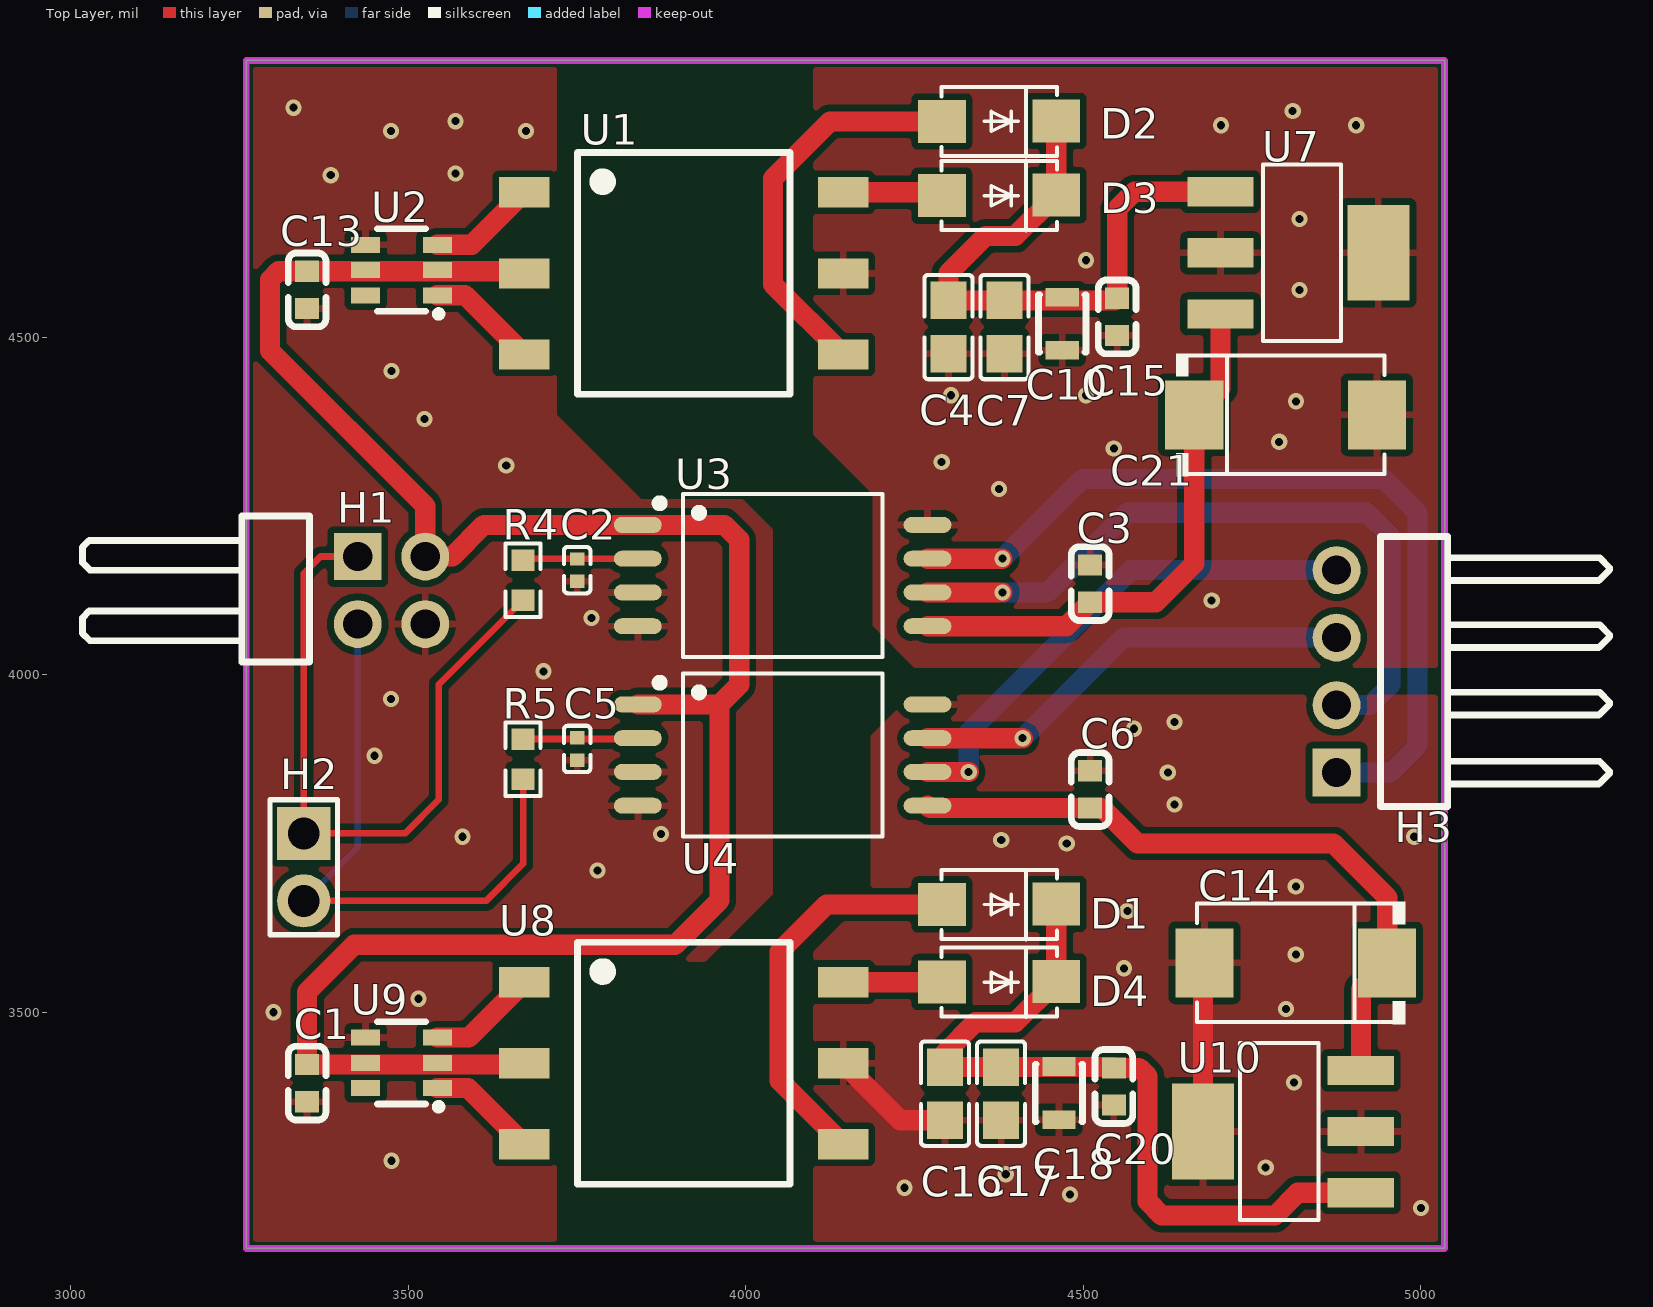
[diagram p0: Top Layer view]
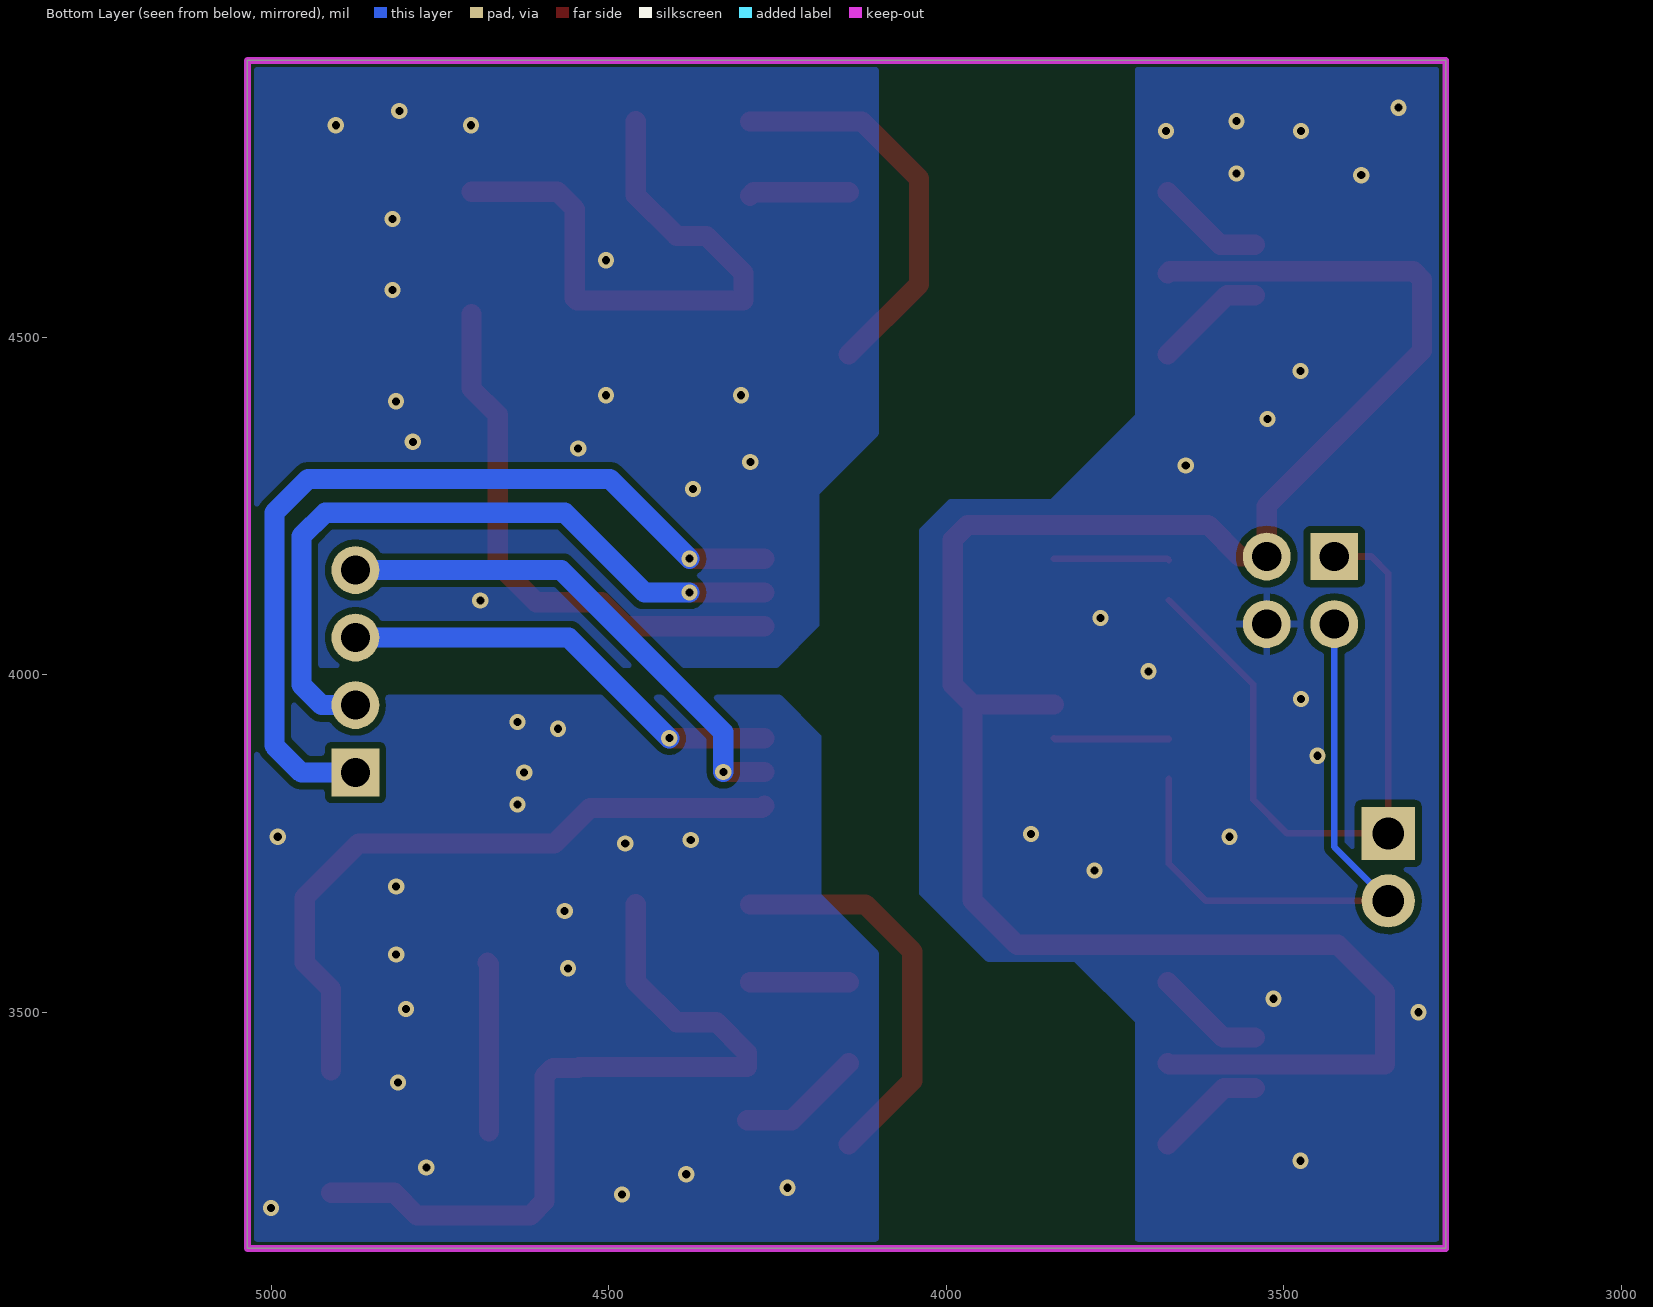
[diagram p1: Bottom Layer view, seen from below]
# Altium PCB MISC51425.pcbdoc
Units mil, origin at the board's own origin, x right, y up, seen from the top; angles counter-clockwise.
Board outline 1775 x 1760 mil, 2 copper layers (Top Layer, Bottom Layer), stack 2.757 mil thick; 33 components, 24 nets, 102 pads, 55 vias.

## Layer stack, top to bottom
Top Solder Mask Layer: solder mask 0.394, Dk 3.3
Top Layer: signal copper 1.379
Bottom Layer: signal copper 1.378
Bottom Solder Mask Layer: solder mask 0.394, Dk 3.3

## Board outline
3260,4910 3260,3150 5035,3150 5035,4910

## Design rules (kind name [scope] priority, off if disabled: settings)
BoardOutlineClearance Plane_innerPlane_1 [All] p2 off: genericclearance=4 ignorepadtopadclearanceinfootprint=FALSE except(0: Arc-SplitContinuation Track-SplitContinuation SMDPad-SplitContinuation THPad-SplitContinuation Via-SplitContinuation Fill-SplitContinuation Region-SplitContinuation Poly-SplitContinuation Text-SplitContinuation Hole-SplitContinuation; 6: Arc-CutoutEdge Track-CutoutEdge SMDPad-CutoutEdge THPad-CutoutEdge Via-CutoutEdge Text-CutoutEdge; 6.9: Hole-OutlineEdge Hole-CutoutEdge; 10: Poly-OutlineEdge Poly-CutoutEdge; 11.8: Arc-OutlineEdge Track-OutlineEdge SMDPad-OutlineEdge THPad-OutlineEdge Via-OutlineEdge Fill-OutlineEdge Region-OutlineEdge Text-OutlineEdge Fill-CutoutEdge Region-CutoutEdge)
BoardOutlineClearance Copper_copperRegion_1 [All] p4 off: genericclearance=4 ignorepadtopadclearanceinfootprint=FALSE except(0: Arc-SplitContinuation Track-SplitContinuation SMDPad-SplitContinuation THPad-SplitContinuation Via-SplitContinuation Fill-SplitContinuation Region-SplitContinuation Poly-SplitContinuation Text-SplitContinuation Hole-SplitContinuation; 6: Arc-CutoutEdge Track-CutoutEdge SMDPad-CutoutEdge THPad-CutoutEdge Via-CutoutEdge Text-CutoutEdge; 6.9: Hole-OutlineEdge Hole-CutoutEdge; 10: Poly-OutlineEdge Poly-CutoutEdge; 11.8: Arc-OutlineEdge Track-OutlineEdge SMDPad-OutlineEdge THPad-OutlineEdge Via-OutlineEdge Fill-OutlineEdge Region-OutlineEdge Text-OutlineEdge Fill-CutoutEdge Region-CutoutEdge)
BoardOutlineClearance copperThickness1oz_1 [All] p6: genericclearance=4 ignorepadtopadclearanceinfootprint=FALSE except(0: Arc-SplitContinuation Track-SplitContinuation SMDPad-SplitContinuation THPad-SplitContinuation Via-SplitContinuation Fill-SplitContinuation Region-SplitContinuation Poly-SplitContinuation Text-SplitContinuation Hole-SplitContinuation; 6: Arc-CutoutEdge Track-CutoutEdge SMDPad-CutoutEdge THPad-CutoutEdge Via-CutoutEdge Text-CutoutEdge; 6.9: Hole-OutlineEdge Hole-CutoutEdge; 10: Poly-OutlineEdge Poly-CutoutEdge; 11.8: Arc-OutlineEdge Track-OutlineEdge SMDPad-OutlineEdge THPad-OutlineEdge Via-OutlineEdge Fill-OutlineEdge Region-OutlineEdge Text-OutlineEdge Fill-CutoutEdge Region-CutoutEdge)
Clearance Plane_innerPlane [All] p1 off: gap=4 ignorepadtopadclearanceinfootprint=FALSE except(6: SMDPad-Track SMDPad-SMDPad THPad-Track SMDPad-THPad THPad-THPad Track-Via SMDPad-Via THPad-Via Via-Via Fill-SMDPad Region-SMDPad Fill-THPad Region-THPad Fill-Via Region-Via Fill-Fill Fill-Region Region-Region Arc-Track Arc-SMDPad Arc-THPad Arc-Via Fill-Arc Region-Arc Arc-Arc Text-Track SMDPad-Text Text-THPad Text-Via Fill-Text Region-Text Arc-Text Text-Text; 6.9: Hole-Track Hole-SMDPad Hole-THPad Hole-Via Fill-Hole Region-Hole Hole-Arc Hole-Text; 10: Poly-Track Poly-SMDPad Poly-THPad Poly-Via Poly-Fill Poly-Region Poly-Poly Poly-Arc Poly-Text Poly-Hole; 11.8: Fill-Track Region-Track)
Clearance Copper_copperRegion [All] p3 off: gap=4 ignorepadtopadclearanceinfootprint=FALSE except(6: SMDPad-Track SMDPad-SMDPad THPad-Track SMDPad-THPad THPad-THPad Track-Via SMDPad-Via THPad-Via Via-Via Fill-SMDPad Region-SMDPad Fill-THPad Region-THPad Fill-Via Region-Via Fill-Fill Fill-Region Region-Region Arc-Track Arc-SMDPad Arc-THPad Arc-Via Fill-Arc Region-Arc Arc-Arc Text-Track SMDPad-Text Text-THPad Text-Via Fill-Text Region-Text Arc-Text Text-Text; 6.9: Hole-Track Hole-SMDPad Hole-THPad Hole-Via Fill-Hole Region-Hole Hole-Arc Hole-Text; 10: Poly-Track Poly-SMDPad Poly-THPad Poly-Via Poly-Fill Poly-Region Poly-Poly Poly-Arc Poly-Text Poly-Hole; 11.8: Fill-Track Region-Track)
Clearance copperThickness1oz [All] p5: gap=4 ignorepadtopadclearanceinfootprint=FALSE except(6: SMDPad-Track SMDPad-SMDPad THPad-Track SMDPad-THPad THPad-THPad Track-Via SMDPad-Via THPad-Via Via-Via Fill-SMDPad Region-SMDPad Fill-THPad Region-THPad Fill-Via Region-Via Fill-Fill Fill-Region Region-Region Arc-Track Arc-SMDPad Arc-THPad Arc-Via Fill-Arc Region-Arc Arc-Arc Text-Track SMDPad-Text Text-THPad Text-Via Fill-Text Region-Text Arc-Text Text-Text; 6.9: Hole-Track Hole-SMDPad Hole-THPad Hole-Via Fill-Hole Region-Hole Hole-Arc Hole-Text; 10: Poly-Track Poly-SMDPad Poly-THPad Poly-Via Poly-Fill Poly-Region Poly-Poly Poly-Arc Poly-Text Poly-Hole; 11.8: Fill-Track Region-Track)
DiffPairsRouting differentialPair [All] p1: maxlimit=6 minlimit=5 mostfreqgap=6 toplayer_minwidth=5 toplayer_prefwidth=100 toplayer_maxwidth=100 toplayer_mingap=5 toplayer_prefgap=6 toplayer_maxgap=6 bottomlayer_minwidth=5 bottomlayer_prefwidth=100 bottomlayer_maxwidth=100 bottomlayer_mingap=5 bottomlayer_prefgap=6 bottomlayer_maxgap=6 maxuncoupledlength=10
HoleToHoleClearance otherClearance [All] p1: gap=11.8 allowstackedmicrovias=TRUE
Length netLength [All] p1: minlimit=0 maxlimit=0
MatchedLengths netLengthTolerance [All] p1: tolerance=1000
PasteMaskExpansion pasteMaskExpansion [All] p1: expansion=0
PlaneConnect innerPlane [All] p1: planeconnectstyle=Relief reliefexpansion=20 reliefentries=4 reliefconductorwidth=10 reliefairgap=10
PolygonConnect copperRegion [(InNet('SGND') OR InNet('$1N9') OR InNet('$1N10'))] p1: connectstyle=Relief reliefconductorwidth=10 reliefentries=4 polygonreliefangle="90 Angle" airgapwidth=10 via.connectstyle=Relief via.reliefconductorwidth=10 via.reliefentries=4 via.polygonreliefangle="90 Angle" via.airgapwidth=10
RoutingVias viaSize [All] p1: holewidth=12.01 width=24.02 viastyle="Through Hole" minholewidth=11.81 minwidth=19.68 maxholewidth=248.03 maxwidth=393.7
SolderMaskExpansion solderMaskExpansion [IsVia] p1: expansion=-1000 istentingtop=TRUE
SolderMaskExpansion solderMaskExpansion [All] p2: expansion=2 istentingtop=FALSE
Width copperThickness1oz_2 [All] p1: maxlimit=100 minlimit=5 preferedwidth=10

## Components (designator, comment, footprint, x,y, rotation, side; value= is the part's Value field where it differs from the comment)
C1 "10uF" C0603 3350,3395 r270 top
C2 "22pF" C0402 3750,4155 r90 top
C3 "100nF" C0603 4510,4135 r270 top
C4 "4.7uF" C0805 4300,4515 r90 top
C5 "22pF" C0402 3750,3890 r90 top
C6 "100nF" C0603 4510,3830 r270 top
C7 "4.7uF" C0805 4383.1,4515 r90 top
C10 "100nF" CAP-SMD_L2.0-W1.25 4468.67,4520 r90 top
C13 "100nF" C0603 3350,4570 r270 top
C14 "47uF" CAP-SMD_L7.3-W4.3-FD 4814.68,3573.21 r180 top
C15 "470nF" C0603 4550,4530 r90 top
C16 "4.7uF" C0805 4295,3379.45 r90 top
C17 "4.7uF" C0805 4378.1,3379.45 r90 top
C18 "100nF" CAP-SMD_L2.0-W1.25 4463.67,3380.18 r90 top
C20 "470nF" C0603 4545,3390 r90 top
C21 "47uF" CAP-SMD_L7.3-W4.3-FD 4799.43,4385 r0 top
D1 "SS34" SMA_L4.3-W2.6-LS5.0-FD 4375,3660 r0 top
D2 "SS34" SMA_L4.3-W2.6-LS5.0-FD 4375,4820 r0 top
D3 "SS34" SMA_L4.3-W2.6-LS5.0-FD 4375,4710 r0 top
D4 "SS34" SMA_L4.3-W2.6-LS5.0-FD 4375,3545 r0 top
H1 "PZ254R-12-4P" HDR-TH_4P-P2.54-H-M-R2-C2-S2.54 3475,4125 r270 top
H2 "PZ254V-11-02P" HDR-TH_2P-P2.54-V-M 3345,3715 r270 top
H3 "PZ254R-11-04P" HDR-TH_4P-P2.54-H-M-W10.4 4875,4005 r90 top
R4 "51Ω" R0603 3670,4140 r90 top
R5 "51Ω" R0603 3670,3875 r90 top
U1 "750342879" XFMR-SMD_6P-L9.1-W8.0-P3.05-LS13.0-TL 3907.91,4594.45 r0 top
U2 "SN6505BDBVR" SOT-23-6_L2.9-W1.6-P0.95-LS2.8-BR 3489.8,4599.45 r0 top
U3 "UCC5350MCQDWVRQ1" SOIC-8_L7.5-W5.9-P1.27-LS11.5-BL 4054.57,4146.89 r270 top
U4 "UCC5350MCQDWVRQ1" SOIC-8_L7.5-W5.9-P1.27-LS11.5-BL 4054.57,3880.97 r270 top
U7 "LM2940IMP-15/NOPB" SOT-223-3_L6.5-W3.4-P2.30-LS7.0-BR 4820,4625 r180 top
U8 "750342879" XFMR-SMD_6P-L9.1-W8.0-P3.05-LS13.0-TL 3907.91,3424.45 r0 top
U9 "SN6505BDBVR" SOT-23-6_L2.9-W1.6-P0.95-LS2.8-BR 3489.8,3425 r0 top
U10 "LM2940IMP-15/NOPB" SOT-223-3_L6.5-W3.4-P2.30-LS7.0-BR 4794.11,3323.21 r0 top

## Footprints (in the part's own frame and the unit in brackets; to place one, negate y for a bottom-side part, rotate by r counter-clockwise, add the part's x,y. Pads: shape width x height; smd on the part's side, far side on the other; paste and mask are expansions set on the pad)
C0402 [mm]
  rect 0.5x0.54 smd: 1(-0.42,0) 2(0.42,0)
  silkscreen extent -0.87,-0.5 0.87,0.5
C0603 [mm]
  rect 0.8x0.9 smd: 1(-0.7,0) 2(0.7,0)
  silkscreen extent -1.39,-0.71 1.39,0.71
C0805 [mm]
  rect 1.41x1.35 smd paste-100 mask+0.051: 1(-1,0) 2(1,0)
  silkscreen extent -1.96,-0.9 1.96,0.9
CAP-SMD_L2.0-W1.25 [mm]
  rect 0.7x1.25 smd: 1(-1,0) 2(1,0)
  silkscreen extent -1.08,-0.89 1.08,0.89
CAP-SMD_L7.3-W4.3-FD [mm]
  rect 2.185x2.592 smd: 1(-3.437,0) 2(3.437,0)
  silkscreen extent -4.11,-2.3 3.72,2.3
HDR-TH_2P-P2.54-V-M [mm]
  rect 2x2 hole 1.2: 1(-1.27,0)
  round 2 hole 1.2: 2(1.27,0)
  silkscreen extent -2.54,-1.27 2.54,1.27
HDR-TH_4P-P2.54-H-M-R2-C2-S2.54 [mm]
  rect 1.778x1.8 hole 1.1: 1(-1.27,-1.27)
  round 1.8 hole 1.1: 2(-1.27,1.27) 3(1.27,-1.27) 4(1.27,1.27)
  silkscreen extent -2.79,-11.63 2.7,-3.09
HDR-TH_4P-P2.54-H-M-W10.4 [mm]
  rect 1.8x1.8 hole 1.1: 1(-3.81,0)
  round 1.8 hole 1.1: 2(-1.27,0) 3(1.27,0) 4(3.81,0)
  silkscreen extent -5.09,-10.27 5.07,-1.65
R0603 [mil]
  rect 31.75x34.02 smd paste-3937.01 mask+2: 1(-29.66,0) 2(29.66,0)
  silkscreen extent -55,-26 55,26
SMA_L4.3-W2.6-LS5.0-FD [mm]
  rect 1.8x1.62 smd: 1(-2.15,-0.009) 2(2.15,0.009)
  silkscreen extent -2.17,-1.32 2.19,1.29
SOIC-8_L7.5-W5.9-P1.27-LS11.5-BL [mm]
  oval 0.6x1.8 smd: 1(-1.905,-5.45) 2(-0.635,-5.45) 3(0.635,-5.45) 4(1.905,-5.45) 5(1.905,5.45) 6(0.635,5.45) 7(-0.635,5.45) 8(-1.905,5.45)
  silkscreen extent -3.06,-4.78 3.06,3.75
SOT-23-6_L2.9-W1.6-P0.95-LS2.8-BR [mm]
  rect 1.1x0.6 smd paste+0 mask+0.051: 1(1.35,-0.95) 2(1.35,0) 3(1.35,0.95) 4(-1.35,0.95) 5(-1.35,0) 6(-1.35,-0.95)
  silkscreen extent -0.9,-1.78 1.52,1.55
SOT-223-3_L6.5-W3.4-P2.30-LS7.0-BR [mm]
  rect 2.5x1.1 smd: 1(2.97,-2.3) 2(2.97,0) 3(2.97,2.3)
  rect 2.34x3.6 smd: 4(-2.97,0)
  silkscreen extent -1.57,-3.33 1.37,3.33
XFMR-SMD_6P-L9.1-W8.0-P3.05-LS13.0-TL [mm]
  rect 1.9x1.14 smd: 1(-6,3.05) 2(-6,0) 3(-6,-3.05) 4(6,3.05) 5(6,0) 6(6,-3.05)
  silkscreen extent -4,-4.55 4,4.55

## Via types
v1: diameter 24.02, hole 12, Top Layer to Bottom Layer, 55 vias

## Nets (pads, with @x,y where several pads share a name; then routed paths per layer and width w, separated by ;. In a path a pad name is that pad's centre, name@x,y a point inside that pad or via, vN(x,y) a via of type N, cw(c..) or ccw(c..) an arc to the next point about the centre after c; other vN are vias at no path point)
15V: C6.2 C14.1 U4.5 U10.3 | length 1009.6
  Top Layer w30: U4.5 4272.67,3802.44 C6.2 4527.56,3802.44 4580,3750 4870,3750 4949.98,3670.02 C14.1 4911.03,3534.26 U10.3
15V_H: C3.2 C21.1 U3.5 U7.3 | length 819.7
  Top Layer w30: U3.5 4474.45,4071.89 C3.2 4607.44,4107.44 4664.13,4164.13 C21.1 4703.07,4423.95 U7.3
$1N9: C4.2 C7.2 C10.2 C15.2 D2.2 D3.2 U7.1 | length 905.5
  Top Layer w30: D2.2 D3.2 4399.27,4650 4355,4650 4300,4595 C4.2 C7.2 4546.81,4554.37 C15.2 4550,4690 4575.55,4715.55 U7.1
$1N10: C16.2 C17.2 C18.2 C20.2 D1.2 D4.2 U10.1 | length 1174
  Top Layer w30: D1.2 D4.2 4399.27,3485 4340,3485 4295,3440 C16.2 C17.2 4543.74,3418.82 C20.2 4582.44,3417.56 4595,3405 4595,3220 4616.21,3198.79 4783.79,3198.79 4817.66,3232.66 U10.1
$1N15: D4.1 U8.4 | length 146.3
  Top Layer w30: U8.4 4290.25,3544.52 D4.1
$1N16: D3.1 U1.4 | length 148.3
  Top Layer w30: U1.4 4285.46,4714.52 D3.1
$1N17: D2.1 U1.6 | length 589.2
  Top Layer w30: U1.6 4040,4578.5 4040,4735 4124.63,4819.63 D2.1
$1N18: D1.1 U8.6 | length 593.8
  Top Layer w30: U8.6 4050,3398.5 4050,3590 4119.63,3659.63 D1.1
$1N21: U1.3 U2.1 | length 165.1
  Top Layer w30: U2.1 3584.02,4562.05 U1.3
$1N22: U8.3 U9.1 | length 163.2
  Top Layer w30: U9.1 3588.47,3387.6 U8.3
$1N25: U8.1 U9.3 | length 162.8
  Top Layer w30: U9.3 3589.57,3462.4 U8.1
$1N26: U1.1 U2.3 | length 160.9
  Top Layer w30: U2.3 3594.02,4636.85 U1.1
$1N41: C2.2 R4.2 U3.2 | length 170.9
  Top Layer w10: R4.2 3672.23,4171.89 U3.2
$1N42: C5.2 R5.2 U4.2 | length 170.5
  Top Layer w10: R5.2 3838.68,3904.66 U4.2
+5V: C1.1 C13.1 H1.2 U1.2 U2.2 U2.5 U3.1 U4.1 U8.2 U9.2 U9.5 | length 3146.2
  Top Layer w30: U8.2 3669.8,3422.56 C1.1 3350,3530 3420,3600 3895,3600 3960.97,3665.97 3960.97,3955.97 ; U1.2 3668.59,4597.56 C13.1 3307.56,4597.56 3295,4585 3295,4480 3525,4250 H1.2 3565,4175 3611.89,4221.89 U3.1 3968.11,4221.89 3990,4200 3990,3985 3960.97,3955.97 ; U4.1 3960.97,3955.97
CLAMP1_H: H3.1 U3.7 | length 1277.1
  Top Layer w30: U3.7 v1(4380,4171.89)
  Bottom Layer w30: v1(4380,4171.89) 4498.11,4290 4945,4290 4995,4240 4995,3895 4955,3855 H3.1
CLAMP1_L: H3.3 U4.7 | length 667.6
  Top Layer w30: U4.7 v1(4410,3905.97)
  Bottom Layer w30: v1(4410,3905.97) 4559.03,4055 H3.3
G1H: H3.2 U3.6 | length 1061.7
  Top Layer w30: U3.6 v1(4380,4121.89)
  Bottom Layer w30: v1(4380,4121.89) 4446.89,4121.89 4565,4240 4920,4240 4955,4205 4955,3985 4925,3955 H3.2
G1L: H3.4 U4.6 | length 764.3
  Top Layer w30: U4.6 v1(4330,3855.97)
  Bottom Layer w30: v1(4330,3855.97) 4330,3915 4570,4155 H3.4
PWM1: H1.1 H2.1 R4.1 | length 1043.2
  Top Layer w10: H1.1 3370,4175 3345,4150 H2.1 3495,3765 3545,3815 3545,3985.34 R4.1
PWM2: H1.3 H2.2 R5.1 | length 916.3
  Top Layer w10: H2.2 3615,3665 3670,3720 R5.1
  Bottom Layer w10: H2.2 3425,3745 H1.3
S1H_0V: C3.1 C4.1 C7.1 C10.1 C15.1 C21.2 U1.5 U3.8 U7.2 U7.4
  other v1: 4690,4110 4375,4275 4290,4315 4545,4335 4790,4345 4815,4405 4304,4414 4504,4414 4820,4570 4504,4614 4820,4675 4704,4814 4904,4814 4810,4835
S1L_0V: C6.1 C14.2 C16.1 C17.1 C18.1 C20.1 U4.8 U8.5 U10.2 U10.4 | length 436.7
  Top Layer w30: U8.5 4228.5,3340.08 C16.1 ; U10.4 4677.18,3571.01 C14.2
  other v1: 5000,3210 4480,3230 4235,3240 4385,3260 4770,3270 4812.05,3395.73 4800,3505 4560,3565 4814.68,3585.36 4565,3650 4814.68,3686.1 4475.32,3750 4378.29,3755.24 4990,3760 4635,3807.58 4625,3855 4575,3920 4635,3930
SGND: C1.2 C2.1 C5.1 C13.2 H1.4 U2.4 U3.3 U3.4 U4.3 U4.4 U9.4
  other v1: 3475,3280 3300,3500 3515,3520 3780,3710 3580,3760 3874.1,3764.1 3450,3880 3474.1,3964.1 3700,4005 3771.34,4084.1 3645,4310 3524.1,4379 3475,4450 3385,4740 3570,4742.4 3474.1,4805.25 3674.1,4805.25 3570,4820 3330,4840
pads on no net: U2.6 U9.6

## Polygon pours and split planes (outlines as drawn)
SGND on Top Layer (solid, remove dead copper, pour order 2): 3130,5010 3640,5010 3720,4930 3720,4385 3845,4260 3995,4260 4040,4215 4040,3675 3940,3575 3810,3575 3720,3485 3720,3095 3625,3000 3110,3000 3000,3110 3000,4880
S1H_0V on Top Layer (solid, remove dead copper, pour order 6): 4100,5040 5090,5040 5127.45,5002.55 5127.45,4074.13 5063.31,4010 4250,4010 4187.91,4072.09 4187.91,4267.55 4100,4355.46
S1L_0V on Top Layer (solid, remove dead copper, pour order 10): 4125,3045 4100,3070 4100,3589.59 4185,3674.59 4185,3910 4245,3970 5056.27,3970 5180.41,3845.86 5180.41,3055.41 5170,3045
SGND on Bottom Layer (solid, remove dead copper, pour order 6): 3130,5010 3640,5010 3720,4930 3720,4385 3845,4260 3995,4260 4040,4215 4040,3675 3940,3575 3810,3575 3720,3485 3720,3095 3625,3000 3110,3000 3000,3110 3000,4880
S1H_0V on Bottom Layer (solid, remove dead copper, pour order 10): 4100,5040 5090,5040 5127.45,5002.55 5127.45,4074.13 5063.31,4010 4250,4010 4187.91,4072.09 4187.91,4267.55 4100,4355.46
S1L_0V on Bottom Layer (solid, remove dead copper, pour order 14): 4125,3045 4100,3070 4100,3589.59 4185,3674.59 4185,3910 4245,3970 5056.27,3970 5180.41,3845.86 5180.41,3055.41 5170,3045

## Keep-outs
Board Outline Layer:
  the board outline again, w10